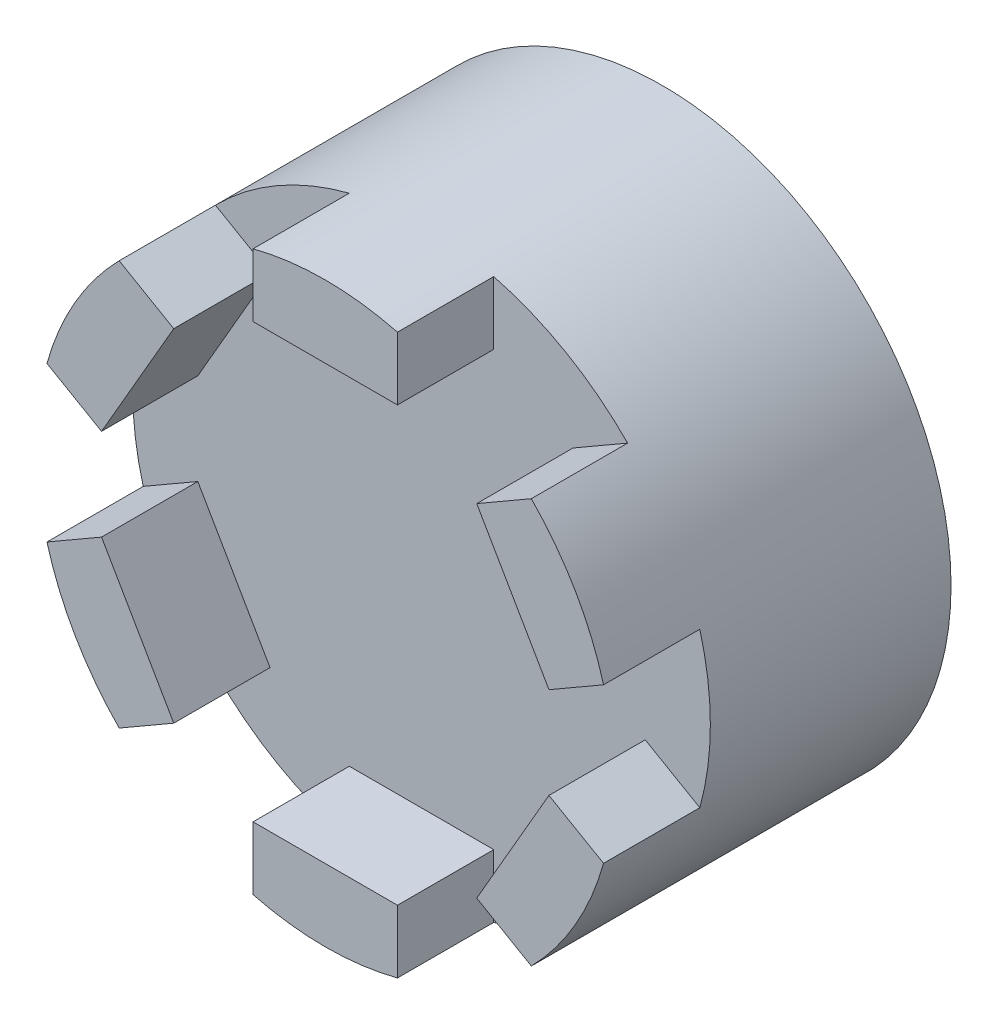
from build123d import *

# Parameters (mm, degrees)
SKETCH_2_R          = 60
EXTRUDE_1_DEPTH     = 50
SKETCH_1_R          = 15
CUT_EXTRUDE_1_DEPTH = 30
EXTRUDE_2_DEPTH     = 20
SKETCH_5_W          = 10
SKETCH_5_H          = 6.88474508
CUT_EXTRUDE_2_DEPTH = 15


with BuildPart() as part:
    # 草图2 → 凸台-拉伸1 (new body)
    with BuildSketch(Plane.XY):
        Circle(SKETCH_2_R)
    extrude(amount=EXTRUDE_1_DEPTH)

    # 草图1 → 切除-拉伸1 (cut)
    with BuildSketch(Plane.XY):
        Circle(SKETCH_1_R)
    extrude(amount=CUT_EXTRUDE_1_DEPTH, mode=Mode.SUBTRACT)

    # 草图3 → 凸台-拉伸2 (add)
    with BuildSketch(Plane.XY.offset(50)):
        with BuildLine():
            Line((42.811529494, 42.037756153), (31.47114317, 35.490381057))
            Line((31.47114317, 35.490381057), (46.47114317, 9.509618943))
            Line((46.47114317, 9.509618943), (57.811529494, 16.05699404))
            ThreePointArc((57.811529494, 16.05699404), (51.961524227, 30), (42.811529494, 42.037756153))
        make_face()
        with BuildLine():
            Line((-15, 58.094750193), (-15, 45))
            Line((-15, 45), (15, 45))
            Line((15, 45), (15, 58.094750193))
            ThreePointArc((15, 58.094750193), (0, 60), (-15, 58.094750193))
        make_face()
        with BuildLine():
            Line((57.811529494, -16.05699404), (46.47114317, -9.509618943))
            Line((46.47114317, -9.509618943), (31.47114317, -35.490381057))
            Line((31.47114317, -35.490381057), (42.811529494, -42.037756153))
            ThreePointArc((42.811529494, -42.037756153), (51.961524227, -30), (57.811529494, -16.05699404))
        make_face()
        with BuildLine():
            Line((15, -58.094750193), (15, -45))
            Line((15, -45), (-15, -45))
            Line((-15, -45), (-15, -58.094750193))
            ThreePointArc((-15, -58.094750193), (0, -60), (15, -58.094750193))
        make_face()
        with BuildLine():
            Line((-42.811529494, -42.037756153), (-31.47114317, -35.490381057))
            Line((-31.47114317, -35.490381057), (-46.47114317, -9.509618943))
            Line((-46.47114317, -9.509618943), (-57.811529494, -16.05699404))
            ThreePointArc((-57.811529494, -16.05699404), (-51.961524227, -30), (-42.811529494, -42.037756153))
        make_face()
        with BuildLine():
            Line((-57.811529494, 16.05699404), (-46.47114317, 9.509618943))
            Line((-46.47114317, 9.509618943), (-31.47114317, 35.490381057))
            Line((-31.47114317, 35.490381057), (-42.811529494, 42.037756153))
            ThreePointArc((-42.811529494, 42.037756153), (-51.961524227, 30), (-57.811529494, 16.05699404))
        make_face()
    extrude(amount=EXTRUDE_2_DEPTH)

    # 草图5 → 切除-拉伸2 (cut)
    with BuildSketch(Plane(origin=(0, 0, 0), x_dir=(-1, 0, 0), z_dir=(0, 0, -1))):
        with Locations((0, 13.55762746)):
            Rectangle(SKETCH_5_W, SKETCH_5_H)
    extrude(amount=-CUT_EXTRUDE_2_DEPTH, mode=Mode.SUBTRACT)


solid = part.part
